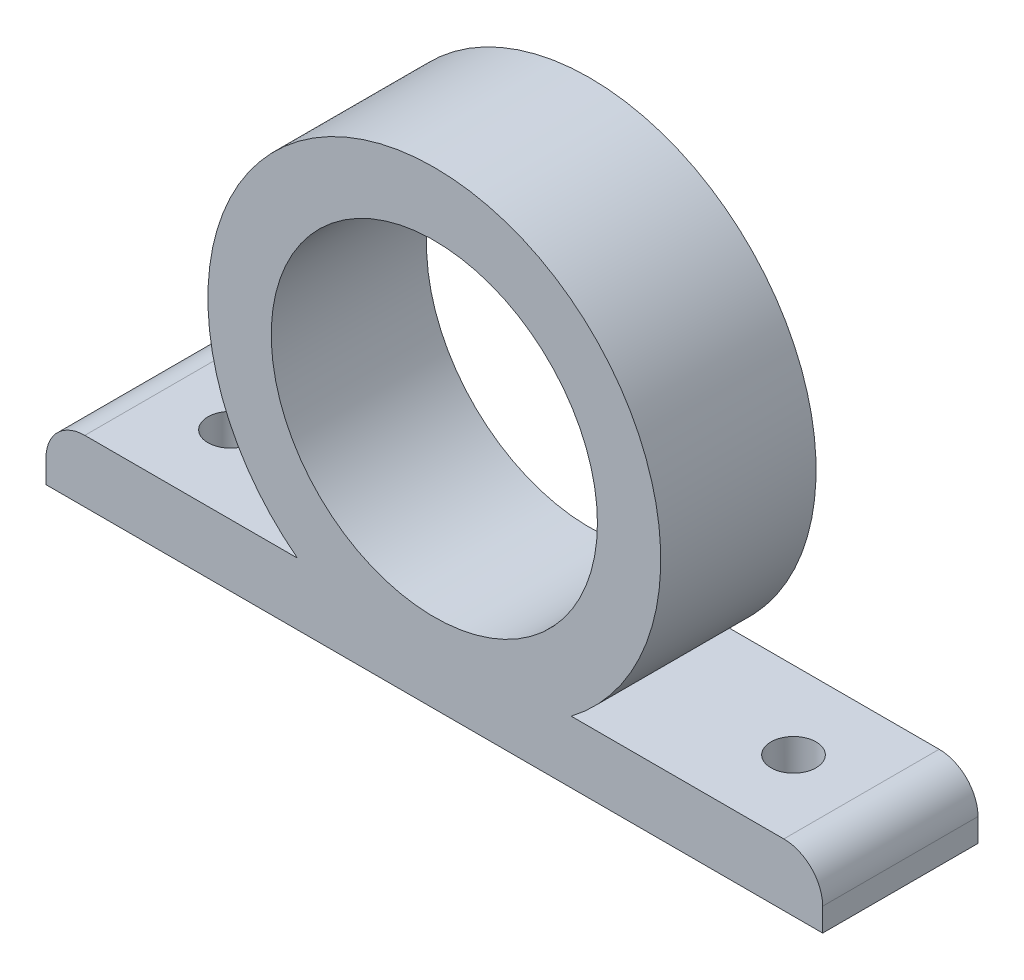
from build123d import *

# Parameters (mm, degrees)
SKETCH1_W           = 100
SKETCH1_H           = 20
BOSS_EXTRUDE1_DEPTH = 8
FILLET1_R           = 5
SKETCH2_R           = 29.154376269
BOSS_EXTRUDE3_DEPTH = 20
SKETCH3_R           = 2.9
CUT_EXTRUDE1_DEPTH  = 26
SKETCH4_R           = 21
CUT_EXTRUDE2_DEPTH  = 74


with BuildPart() as part:
    # Sketch1 → Boss-Extrude1 (new body)
    with BuildSketch(Plane(origin=(0, 0, 0), x_dir=(1, 0, 0), z_dir=(0, 1, 0))):
        Rectangle(SKETCH1_W, SKETCH1_H)
    extrude(amount=BOSS_EXTRUDE1_DEPTH)

    # Fillet1
    fillet1_edges = [part.edges().sort_by_distance(p)[0] for p in [
        (-50, 8, 0),
        (50, 8, 0),
    ]]
    fillet(fillet1_edges, radius=FILLET1_R)

    # Sketch2 → Boss-Extrude3 (add)
    with BuildSketch(Plane.XY.offset(10)):
        with Locations((0, 31.226436769)):
            Circle(SKETCH2_R)
    extrude(amount=-BOSS_EXTRUDE3_DEPTH)

    # Sketch3 → Cut-Extrude1 (cut)
    with BuildSketch(Plane(origin=(0, 8, 0), x_dir=(1, 0, 0), z_dir=(0, 1, 0))):
        with Locations(Location((-36.246581996, 0, 0), (0, 0, 270))):
            Circle(SKETCH3_R)
        with Locations(Location((36.246581996, 0, 0), (0, 0, 270))):
            Circle(SKETCH3_R)
    extrude(amount=-CUT_EXTRUDE1_DEPTH, mode=Mode.SUBTRACT)

    # Sketch4 → Cut-Extrude2 (cut)
    with BuildSketch(Plane.XY.offset(10)):
        with Locations((0, 31.226436769)):
            Circle(SKETCH4_R)
    extrude(amount=-CUT_EXTRUDE2_DEPTH, mode=Mode.SUBTRACT)


solid = part.part
